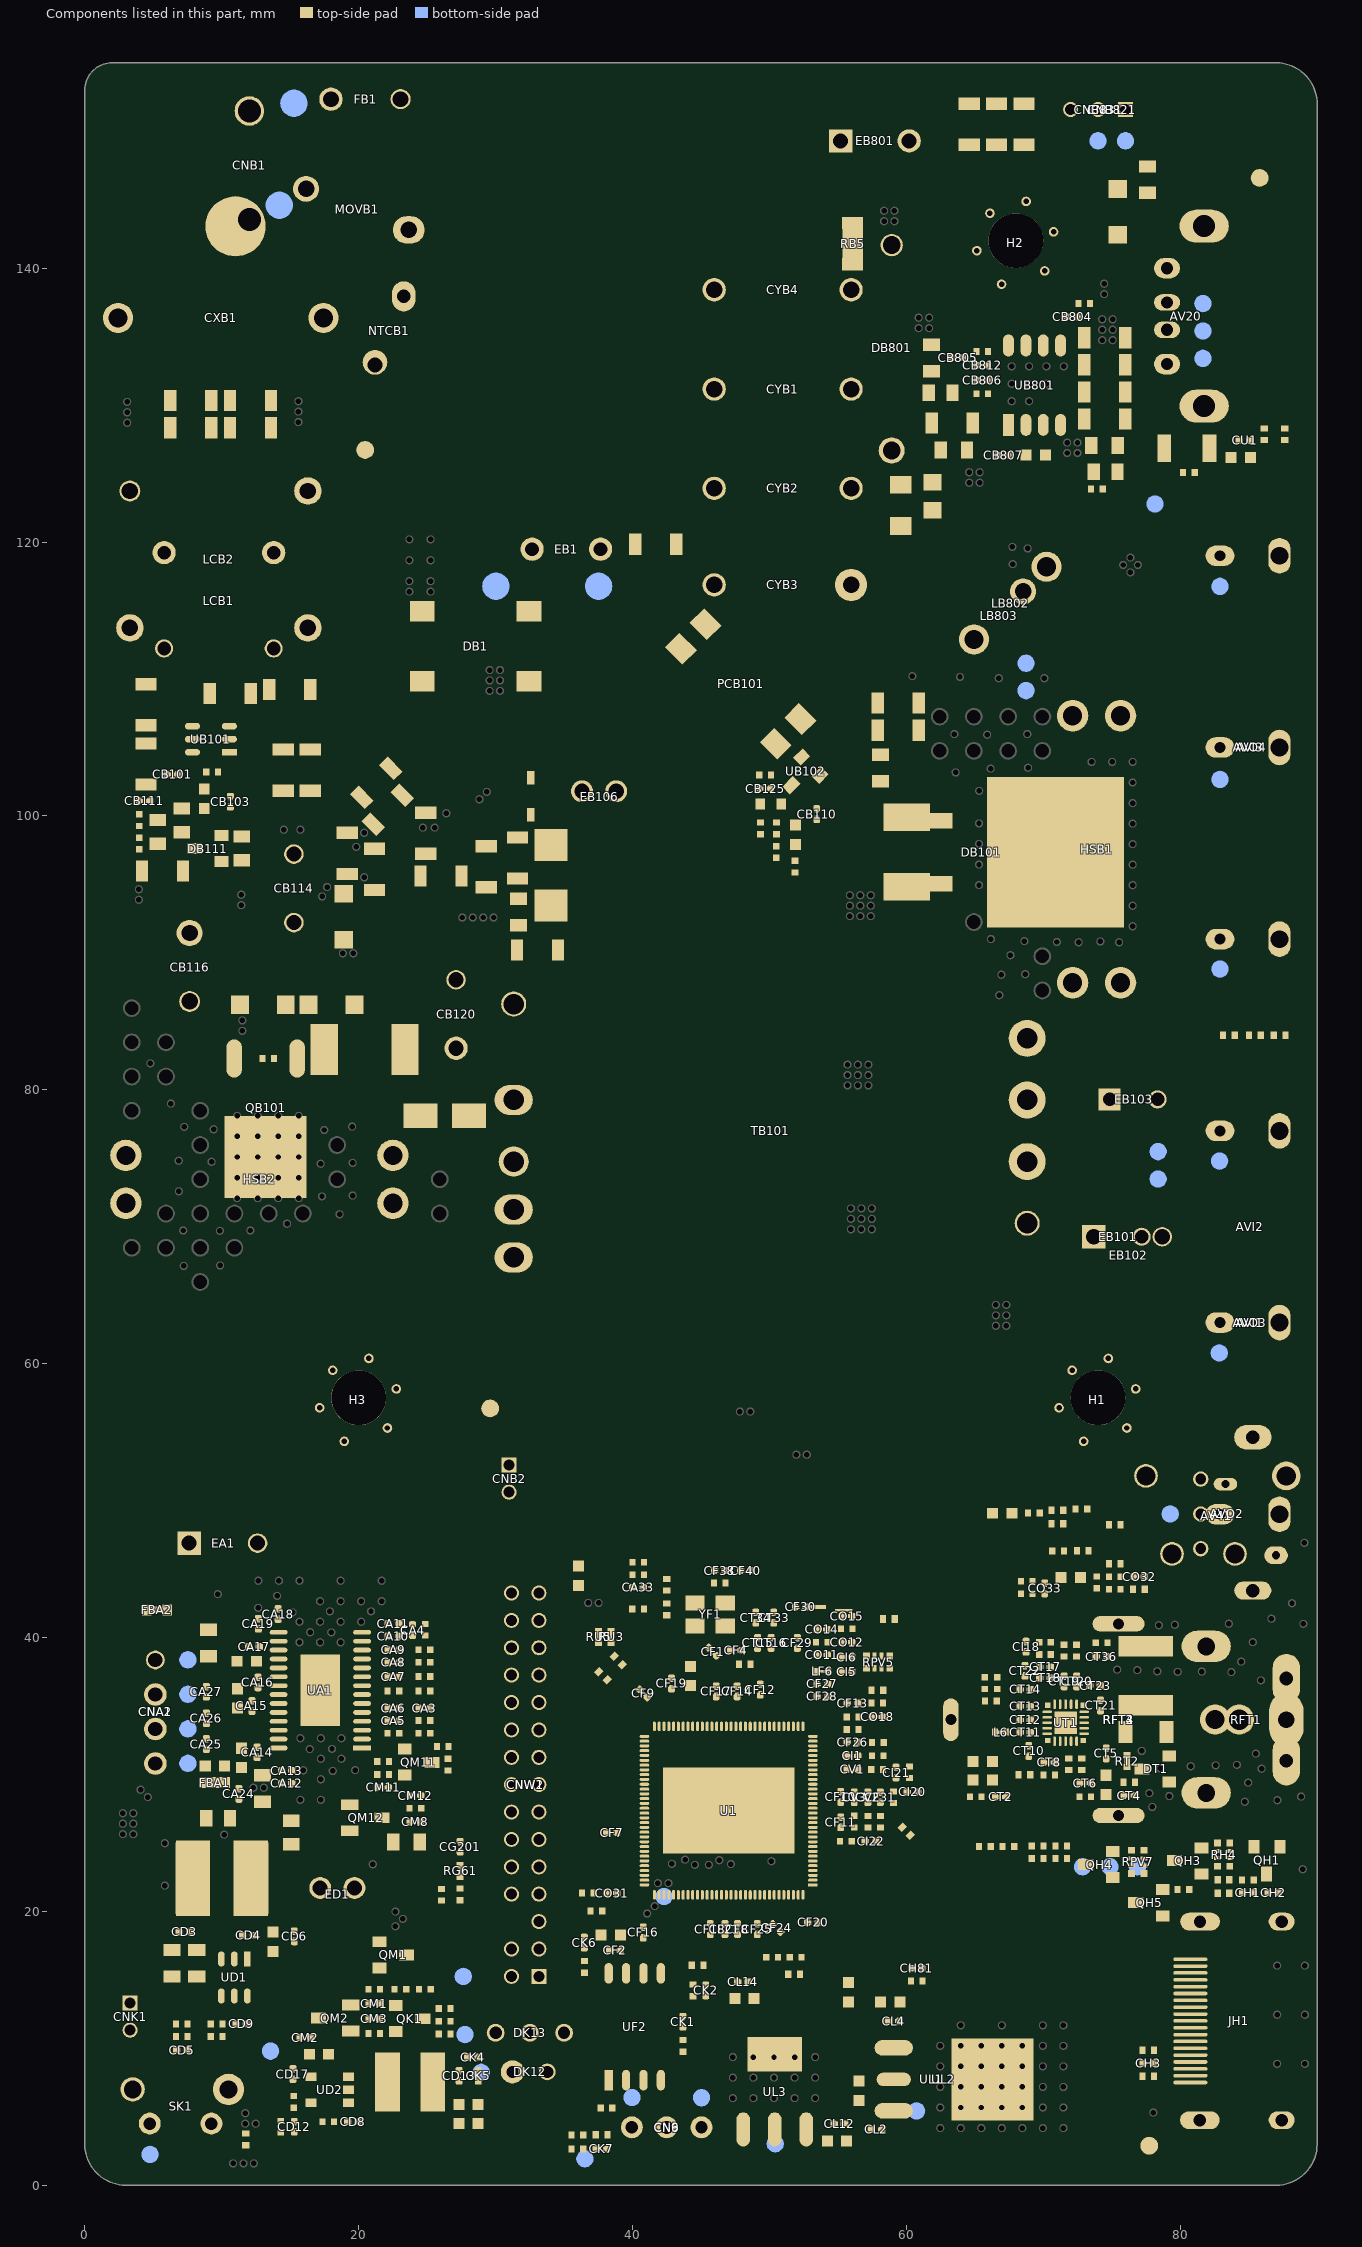
[diagram p0: the components of this part, seen from the top]
# Altium PCB MISC116569.PcbDoc (part 15 of 15)
Units mm, origin at the board's own origin, x right, y up, seen from the top; angles counter-clockwise.
Board outline 90 x 155 mm, 2 copper layers (TopLayer, BottomLayer), stack 1.571 mm thick; 527 components, 277 nets, 2450 pads, 649 vias.

## Silkscreen, mask and mechanical layers (free items; w line width, h text height) (continued)
BottomOverlay:
  circle w0.15: c26.602,150.76 r0.051
  circle w0.102: c26.602,151.913 r0.051
  circle w0.102: c7.743,125.916 r0.051
  circle w0.15: c7.743,124.763 r0.051
  circle w0.102: c7.768,129.878 r0.051
  circle w0.15: c7.768,128.726 r0.051
  circle w0.102: c12.149,125.929 r0.051
  circle w0.15: c12.149,124.776 r0.051
  circle w0.102: c12.188,129.878 r0.051
  circle w0.15: c12.188,128.726 r0.051
  circle w0.102: c20.827,81.656 r0.051
  circle w0.15: c20.827,80.504 r0.051
  rectangle: 288.542,45.77 291.849,47.77
  lines w0.127: 7.704,125.915 7.743,125.116 7.781,125.915 ; 7.73,129.878 7.768,129.078 7.806,129.878 ; 12.111,125.928 12.149,125.129 12.188,125.928 ; 12.149,129.878 12.188,129.078 12.226,129.878 ; 20.789,81.656 20.827,80.856 20.865,81.656 ; 26.564,151.912 26.602,151.113 26.64,151.912 ; 302.535,45.77 302.535,47.77 ; 6.401,124.473 9.001,124.473 7.751,126.423 6.401,124.473 ; 6.426,128.435 9.026,128.435 7.776,130.385 6.426,128.435 ; 10.808,124.485 13.408,124.485 12.158,126.435 10.808,124.485 ; 10.846,128.435 13.446,128.435 12.196,130.385 10.846,128.435 ; 19.485,80.213 22.085,80.213 20.835,82.163 19.485,80.213 ; 25.26,150.47 26.61,152.42 27.86,150.47 25.26,150.47 ; 77.214,6.747 87.714,6.747 87.714,17.247 77.214,17.247 77.214,6.747 ; 288.542,45.77 288.542,47.77 307.135,47.77 307.135,45.77 288.542,45.77
  lines w0.2: 4.483,10.274 7.912,10.274 7.912,14.516 4.508,14.516 ; 4.572,29.566 0.445,29.566 0.445,39.573 4.724,39.573
  lines w0.3: 70.383,119.964 69.901,119.964 ; 70.853,152.679 70.853,154.724 75.044,154.724 77.127,154.724 77.127,152.692 ; 71.629,153.848 72.454,153.848 ; 73.629,153.848 74.454,153.848 ; 75.628,153.848 76.454,153.848 ; 76.035,153.441 76.035,154.267 ; 80.734,50.203 84.214,50.203 ccw(c84.214,50.775) 84.785,50.775 84.785,51.968 ccw(c84.087,51.968) 84.087,52.667 82.182,52.667 ; 69.901,119.964 70.815,119.964 70.929,119.85 71.971,118.808 71.971,118.415 71.971,117.907 68.834,114.77 68.301,114.77 66.84,116.23 66.84,116.903 68.11,118.173 69.901,119.964 ; 1.198,71.688 ccw(c2.988,71.681) 4.776,71.769 4.776,75.094 ccw(c2.988,75.181) 1.198,75.175 1.198,71.688 ; 8.287,140.836 8.674,140.449 16.777,140.449 17.539,141.211 17.539,146.444 16.878,147.104 8.941,147.104 8.287,146.45 8.287,142.228 8.287,140.836 ; 9.398,149.606 10.173,148.831 18.11,148.831 19.279,150 19.279,154 18.771,154.508 13.665,154.508 10.071,154.508 9.398,153.835 9.398,149.606 ; 20.698,71.688 ccw(c22.488,71.681) 24.276,71.769 24.276,75.094 ccw(c22.488,75.181) 20.698,75.175 20.698,71.688 ; 72.148,89.611 ccw(c72.141,87.82) 72.228,86.032 75.554,86.032 ccw(c75.641,87.82) 75.634,89.611 72.148,89.611 ; 72.148,109.111 ccw(c72.141,107.321) 72.228,105.532 75.554,105.532 ccw(c75.641,107.321) 75.634,109.111 72.148,109.111 ; 77.953,45.39 ccw(c78.727,45.39) 78.727,44.615 83.566,44.615 84.252,44.615 ccw(c84.252,45.885) 85.522,45.885 85.522,46.558 ccw(c84.418,46.558) 84.418,47.662 78.479,47.662 ccw(c78.479,47.136) 77.953,47.136 77.953,45.39
  lines w0.5: 0.394,56.896 11.973,56.896 18.476,63.398 23.8,63.398 26.937,60.261 38.824,60.261 47.583,69.021 47.583,106.029 53.806,112.252 53.806,143.473 48.434,148.845 48.434,154.623 43.434,154.623 43.434,146.774 48.806,141.402 48.806,114.323 42.583,108.1 42.583,71.092 36.753,65.262 29.008,65.262 25.871,68.398 16.405,68.398 9.902,61.896 0.394,61.896 0.394,56.896
  text "FB1" at 27.381,152.806 h1.27
  text "USB IN" at 88.003,133.703 h1.52 r270
  text "AV OUT" at 78.245,100.305 h1.52
  text "YPBPR IN" at 78.245,98.704 h1.52
  text "AUDIO IN" at 89.332,70.396 h1.52
  text "CVBS IN" at 89.484,60.134 h1.52
  text "COAX OUT" at 89.484,58.788 h1.52
  text "OPTICAL OUT" at 89.484,57.442 h1.52
  text "EARPHONE OUT" at 89.484,56.096 h1.52
  text ".GBO" at 303.163,46.355 h1.52
  text "BottomOverlay" at 292.452,46.33 h1.52
  text "RF IN" at 89.014,26.924 h1.52
  text "GND" at 7.397,12.892 h1.27
  text "KEY" at 7.397,10.889 h1.27
  text "HDMI(ARC) IN" at 87.265,2.316 h1.52
TopPaste:
  rectangle: 288.542,63.382 291.849,65.382
  lines w0.127: 302.535,63.382 302.535,65.382 ; 288.542,63.382 307.135,63.382 307.135,65.382 288.542,65.382 288.542,63.382
  text "TopPaste" at 292.744,63.922 h1.52
  text ".GTP" at 303.147,63.868 h1.52
BottomPaste:
  rectangle: 288.542,43.378 291.849,45.378
  lines w0.127: 302.535,43.378 302.535,45.378 ; 288.542,43.378 307.135,43.378 307.135,45.378 288.542,45.378 288.542,43.378
  text "BottomPaste" at 292.423,43.962 h1.52
  text ".GBP" at 303.17,43.832 h1.52
TopSolder:
  rectangle: 288.542,58.558 291.849,60.558
  lines w0.127: 302.535,58.558 302.535,60.558 ; 288.542,58.558 307.135,58.558 307.135,60.558 288.542,60.558 288.542,58.558
  text "TopSolder" at 292.757,59.068 h1.52
  text ".GTS" at 303.147,59.026 h1.52
BottomSolder:
  drawing of 29 lines, arcs and shapes, not listed
  text "BottomSolder" at 292.423,48.697 h1.52
  text ".GBS" at 303.146,48.674 h1.52
过炉治具:
  circle w0.025: c6.833,109.474 r1.55
  circle w0.025: c16.205,106.895 r1.55
  circle w0.025: c6.515,108.242 r1.55
  circle w0.025: c20.879,107.378 r1.55
  lines w0.5: 21.895,103.708 27.064,103.708 ; 27.064,103.759 28.067,104.762 33.033,104.762 ; 33.075,99.301 36.046,99.301 ; 33.731,90.843 33.731,91.719 34.239,92.227 34.887,92.227 35.814,91.3 ; 34.237,90.261 36.338,88.16 ; 34.265,98.451 36.366,100.552 ; 36.202,94.939 38.303,97.041 ; 36.538,83.058 36.538,86.03
  lines w1.5: 2.807,104.076 5.779,104.076 6.02,104.318 6.02,107.277 ; 10.617,110.846 10.617,108.153 11.074,107.696 15.253,107.696 ; 11.614,112.122 13.119,110.617 15.342,110.617
  lines w2: 47.684,90.424 63.978,90.424 64.524,89.878 ; 59.563,72.149 59.563,90.221 ; 63.69,71.819 63.69,89.891
  lines w2.1: 12.04,102.171 12.04,100.457 13.116,99.381 13.116,92.98 ; 13.271,90.183 13.271,93.154 ; 13.58,103.318 20.443,103.318 20.853,102.908 ; 13.64,89.281 17.92,89.281 19.126,88.075 21.666,88.075 ; 17.332,93.716 17.332,99.654 18.313,100.635 18.313,102.438 ; 24.238,102.927 25.362,101.803 27.394,101.803 28.727,103.137 31.242,103.137 ; 26.302,91.986 26.302,93.523 31.001,98.222 ; 26.429,86.157 22.454,90.132 22.454,94.805 27.343,99.695 ; 26.645,91.249 28.981,91.249 31.686,88.544 32.614,88.544 33.909,87.249 33.909,85.712 ; 27.33,101.422 27.33,106.566 28.816,108.052 ; 29.756,107.658 32.728,107.658 ; 31.623,112.776 34.595,112.776 ; 34.531,108.394 34.531,114.96
  lines w3.1: 4.293,109.664 5.804,109.664 10.655,104.813 ; 21.915,115.773 21.915,124.193 26.373,128.651 48.598,128.651 ; 23.101,133.731 48.865,133.731
  lines w3.2: 14.734,148.539 23.116,148.539
  lines w5: 65.476,122.885 73.858,122.885
  lines w8: 28.672,62.598 35.796,62.598 44.763,71.564 44.763,106.083 50.871,112.192 50.871,142.049 48.306,144.615 48.306,157.404
3D和装配:
  lines w0.127: 75.714,5.247 75.714,18.747 89.214,18.747 89.214,5.247 75.714,5.247
  lines w3.1: 18.842,124.028 24.503,124.028 29.332,119.199 29.332,113.093 ; 19.972,106.578 19.972,121.069
  text "2L,4,90.00×155.00mm,FR4(TG130-CTI175),1OZ,Green,OSP,1.6mm,6,72,77.5%,12.93,0.4mm" at 292.816,174.588 h1.52
自动测试:
  circle w0.076: c1.215,20.845 r5
  circle w0.076: c0.301,84.726 r5
  circle w0.076: c47.253,149.915 r5
  circle w0.076: c43.697,95.178 r5
  circle w0.076: c84.857,150.169 r5
  circle w0.076: c5.203,60.278 r5
  circle w0.076: c67.966,17.416 r5
  circle w0.076: c55.114,48.556 r5
顶层限制:
  drawing of 3667 lines, arcs and shapes, not listed
  text "22" at 76.917,159.014 h2.5
  text "L" at 13.078,147.06 h2 r90
  text "AC IN" at 13.999,138.527 h1.27 r90
  text "AC IN" at 16.382,138.093 h1.27 r90
  text "N" at 13.038,132.157 h2 r90
  text "Heat dissipation air duct" at 37.912,91.141 h6
  text "AC" at -31.59,71.669 h5.08
  text "149" at 142.735,71.585 h2.5 r90
  text "142" at 136.735,68.085 h2.5 r90
  text "A hole" at 18.324,65.028 h2
  text "A hole" at 71.557,65.028 h2
  text "136.5" at 130.735,63.668 h2.5 r90
  text "8.5" at 172.462,57.661 h2.5 r180
  text "1.9" at 180.209,50.27 h2.5 r180
  text "105" at 124.735,49.792 h2.5 r90
  text "9.5" at 164.715,47.349 h2.5 r90
  text "11.4" at 161.673,45.349 h2.5 r180
  text "SPEAKER" at 3.29,45.08 h1.52
  text "6" at 179.523,44.58 h2.5 r180
  text "30" at 24.662,43.914 h1.27 r270
  text "29" at 30.932,43.899 h1.27 r270
  text "19" at 31.072,34.061 h1.27 r270
  text "20" at 24.633,34.031 h1.27 r270
  text "63" at 119.985,29.417 h2.5 r90
  text "LVDS" at 33.262,29.091 h1.52
  text "57.5" at 116.286,25.001 h2.5 r90
  text "9" at 30.935,24.079 h1.27 r270
  text "10" at 24.629,23.972 h1.27 r270
  text "12.8" at 93.067,23.734 h2.5
  text "49" at 111.68,22.417 h2.5 r90
  text "2" at 24.671,16.129 h1.27 r270
  text "34" at 106.735,14.917 h2.5 r90
  text "12" at 100.735,4.333 h2.5 r90
  text "16" at 80.333,-7.42 h2.5
  text "1.85" at -6.789,-8.1 h2.5
  text "47.51" at 61.664,-13.42 h2.5
  text "57.5" at 57.502,-19.42 h2.5
  text "70" at 53.125,-25.42 h2.5
  text "83" at 46.415,-31.42 h2.5
  text "90" at 43.124,-37.42 h2.5
  text "3.85" at 31.932,-46.586 h1.27
  text "3.85" at 31.932,-46.586 h1.27
  text "1.6" at 89.671,-47.561 h2.5
  text "2.92" at 33.734,-52.286 h1.27 r315
  text "2.92" at 33.932,-52.461 h1.27 r315
  text "3.6" at 31.157,-52.986 h1.27 r90
  text "3.6" at 31.157,-52.986 h1.27 r90
  text "1.94" at 16.594,-57.561 h2.5
  text "IR" at 39.813,-64.307 h3
  text "5.55" at 38.317,-64.511 h2.5 r90
  text "LED" at 28.147,-64.615 h3
  text "KEY" at 4.439,-65.128 h3
底层限制:
  circle w0.127: c74,57.502 r2
  circle w0.127: c20,57.502 r2
  circle w0.127: c68,142.004 r2
  circle w0.127: c68,142.004 r6
  circle w0.127: c20,57.502 r6
  circle w0.127: c20,57.502 r8
  circle w0.127: c74,57.502 r8
  circle w0.127: c68,142.004 r8
  circle w0.127: c20,57.502 r13
  lines w0.127: -10.001,3 ccw(c-7.001,3) -7.001,0 2.998,0 87,0 ccw(c87,3) 90,3 90,146.002 ; -10,3.002 -10,152.003 cw(c-7,152.003) -7,155.003 87,155.003 cw(c87,152.003) 90,152.003 90,146.002 ; 3,0 cw(c3,3) 0,3 0,146.002 cw(c3,146.002) 3,149.002 87,149.002 cw(c87,146.002) 90,146.002
附加说明:
  lines w0.127: 391.994,170.329 420.696,170.329 ; 391.994,173.056 420.696,173.056 ; 391.994,175.782 420.696,175.782 ; 391.994,178.508 420.696,178.508 ; 391.994,181.234 428.329,181.234 ; 399.627,167.603 399.627,183.961 ; 420.696,167.603 420.696,183.961 ; 429.675,170.329 479.675,170.329 ; 429.675,173.056 479.675,173.056 ; 429.675,175.782 479.675,175.782 ; 429.675,178.508 479.675,178.508 ; 429.675,181.234 479.675,181.234 ; 432.329,167.603 432.329,181.234 ; 391.994,167.603 428.329,167.603 428.329,183.961 391.994,183.961 391.994,167.603 ; 429.675,167.603 429.675,183.961 479.675,183.961 479.675,167.603 429.675,167.603
  text "Keep descriptions concise so derived projects or board revisions can inherit them:" at 439.945,182.818 h0.89
  text "Template date:" at 336.212,182.132 h1.52
  text "Version/cycle number" at 392.549,182.103 h1.52
  text "Customer" at 423.499,182.103 h1.52
  text "Special remark information" at 430.471,182.103 h1.52
  text "PCB designer" at 406.659,182.09 h1.52
  text "2019.10.12" at 344.391,182.043 h1.52
  text "If new or special design rules apply: Bangladesh hole spacing; special safety clearance; special stack-up that must not change; support chain; designated factory..." at 439.933,181.662 h0.89
  text "Board utilization:" at 336.199,179.668 h1.52
  text "8X%" at 344.391,179.567 h1.52
  text "(Fill in for non-TV business unit projects)" at 349.217,179.567 h1.52
  text "This project requires shipment to Bangladesh" at 433.189,179.554 h0.89
  text "XXXXXX" at 393.044,179.385 h1.52
  text "1" at 430.725,179.385 h1.52
  text "CK" at 400.766,179.364 h1.52
  text "2" at 430.724,176.663 h1.52
  text "3" at 430.725,173.945 h1.52
  text "COMPANY_A" at 423.583,173.888 h1.52
  text "4" at 430.725,171.202 h1.52
  text "① Panel production, single-board shipment" at 321.835,170.321 h0.76
  text "Special board requirements; leave blank if none;" at 300.402,169.492 h1.52
  text "Reference:" at 318.406,169.47 h1.52
  text "② 4-up panel production, 2-up shipment" at 321.823,169.204 h0.76
  text "5" at 430.725,168.484 h1.52
  text "The remark items below must be copied to the TopOverlay layer; one or two items may be remarked" at 325.734,103.938 h1.52
  text "Only one barcode position on the board; the other barcode must be stuck on a component" at 364.308,103.865 h1.52
  text "No barcode position on the board; the barcode must be stuck on a component" at 364.308,101.853 h1.52
  text "Customer special requirements; special process requirements; leave blank if none" at 307.778,98.986 h1.52
  text "Height value and reference designator of SMD components over 2mm on the solder side; leave blank if none" at 307.778,96.446 h1.52
  text "Reference designator of easily damaged components; leave blank if none" at 307.733,92.734 h1.52
  text "Reference designator of new footprints; leave blank if none" at 307.793,87.475 h1.52
  text "Suction cup and press bar positions are reserved: enter 'Yes', otherwise enter 'No'" at 307.815,82.323 h1.52
  text "X.XXXX.XXX Stencil Revision Explanation" at 284.339,33.781 h1.52
  text "X.XXXX.XXX Testing jig Revision Explanation" at 284.326,32.029 h1.52
  text "X.XXXX.XXX Wave-soldering jig Revision Explanation" at 284.313,30.301 h1.52
DrillDrawing:
  text ".Legend" at 284.467,185.186 h1.52